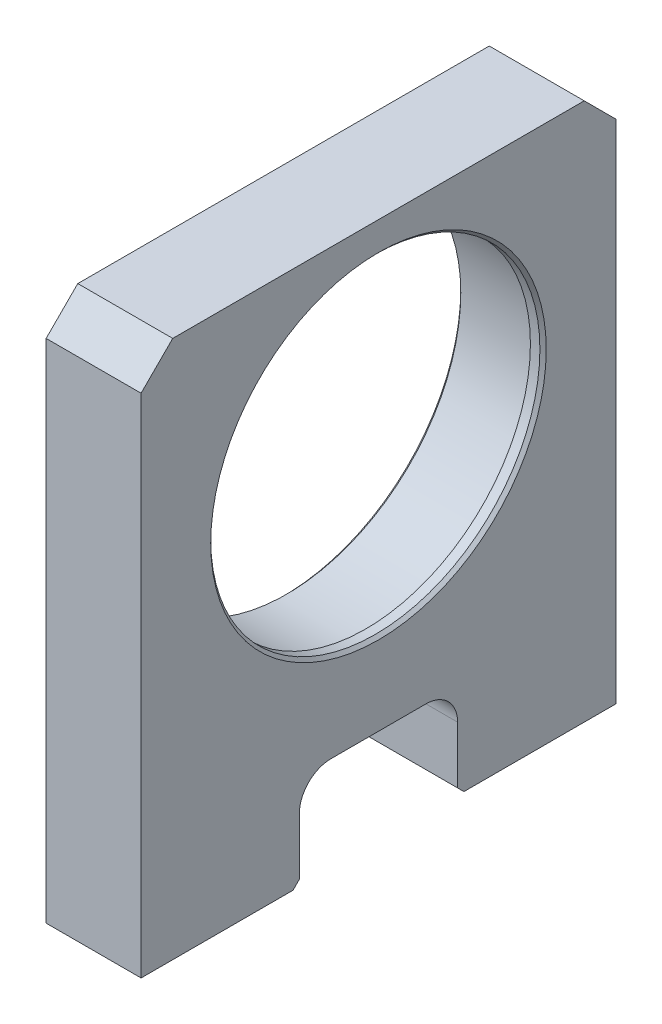
SolidWorks part; units mm, degrees
material "S45C"
ref_plane "Front Plane" through (0, 0, 0) normal (0, 0, 1) x (1, 0, 0)
ref_plane "Top Plane" through (0, 0, 0) normal (0, 1, 0) x (1, 0, 0)
ref_plane "Right Plane" through (0, 0, 0) normal (1, 0, 0) x (0, 0, -1)
sketch "Sketch1" plane through (0, 0, 0) normal (1, 0, 0) x (0, 0, -1)
  line L0 (0, 0) -> (0, -69.2188) construction
  line L1 (-37.5, -42.5) -> (-12.5, -42.5)
  line L2 (-37.5, -42.5) -> (-37.5, 42.5)
  line L3 (-37.5, 42.5) -> (37.5, 42.5)
  line L4 (37.5, -42.5) -> (37.5, 42.5)
  line L5 (-37.5, -42.5) -> (37.5, 42.5) construction
  line L6 (-37.5, 42.5) -> (37.5, -42.5) construction
  line L8 (-12.5, -42.5) -> (-12.5, -32.5)
  line L9 (-7.5, -27.5) -> (7.5, -27.5)
  line L10 (12.5, -42.5) -> (12.5, -32.5)
  line L11 (12.5, -42.5) -> (37.5, -42.5)
  circle A0 centre (0, 11.5) radius 27.5
  arc A1 (-12.5, -32.5) -> (-7.5, -27.5) centre (-7.5, -32.5) cw
  arc A2 (7.5, -27.5) -> (12.5, -32.5) centre (7.5, -32.5) cw
  point P0 (0, 0)
  point P16 (-12.5, -27.5)
  point P19 (12.5, -27.5)
  dimension "D3" = 54
  dimension "D4" = 55
  dimension "D7" = 5
  dimension "D1" = 75
  dimension "D2" = 85
  dimension "D5" = 25
  dimension "D6" = 15
extrude "Boss-Extrude2" add sketch "Sketch1" along normal mid plane 15
hole_wizard "M6 Tapped Hole1" positions "Sketch3" profile "Sketch2" tap size "M6" standard "Gb"
sketch "Sketch3" plane through (0, -42.5, 0) normal (0, -1, 0) x (-1, 0, 0)
  line L3 (43.4921, 0) -> (-42.8148, 0) construction
  point P0 (0, -32.5)
  point P2 (0, 32.5)
  dimension "D1" = 65
sketch "Sketch2" plane through (0, -42.5, 32.5) normal (1, 0, 0) x (0, 0, -1)
  line L0 (0, 0) -> (0, 18.5022)
  line L1 (0, 18.5022) -> (2.5, 17)
  line L2 (2.5, 17) -> (2.5, 0)
  line L5 (2.5, 0) -> (0, 0)
  line L10 (0, 18.5022) -> (-2.5, 17) construction
  line L11 (0, -6.35) -> (0, 107.95) construction
  dimension "螺纹孔钻头直径" = 5
  dimension "螺纹孔钻头深度" = 17
  dimension "导头角度" = 118
cosmetic thread "Cosmetic Thread1" parameters "D1"=12, "D2"=6
cosmetic thread "Cosmetic Thread2" parameters "D1"=12, "D2"=6
sketch "Sketch5" plane through (7.5, 0, 0) normal (1, 0, 0) x (0, 0, -1)
  circle A0 centre (0, 11.5) radius 27.5
  circle A1 centre (0, 11.5) radius 26
  circle A2 centre (0, 11.5) radius 27.5 construction
  dimension "D1" = 52
extrude "Boss-Extrude3" add sketch "Sketch5" against normal blind 2
chamfer "Chamfer1" distance 5 angle 45 2 edges at (0, 42.5, -37.5) (0, 42.5, 37.5)
sketch "Sketch4" plane through (0, -42.5, 0) normal (0, -1, 0) x (1, 0, 0)
  line L0 (26.9042, 0) -> (-24.8554, 0) construction
  line L1 (0, 20.5) -> (0, 19.5) construction
  line L2 (2.5, 20.5) -> (2.5, 19.5)
  line L3 (-2.5, 20.5) -> (-2.5, 19.5)
  circle A0 centre (0, -20) radius 2.5
  arc A1 (2.5, 20.5) -> (-2.5, 20.5) centre (0, 20.5) ccw
  arc A2 (-2.5, 19.5) -> (2.5, 19.5) centre (0, 19.5) ccw
  point P7 (0, 20)
  dimension "D1" = 40
  dimension "D2" = 5
  dimension "D3" = 1
extrude "Cut-Extrude1" cut sketch "Sketch4" against normal blind 15
chamfer "Chamfer2" distance 1 angle 45 2 edges at (0, -42.5, 12.5) (0, -42.5, -12.5)
chamfer "Chamfer3" distance 0.5 angle 45 2 edges at (-7.5, 11.5, -27.5) (7.5, 11.5, -26)
